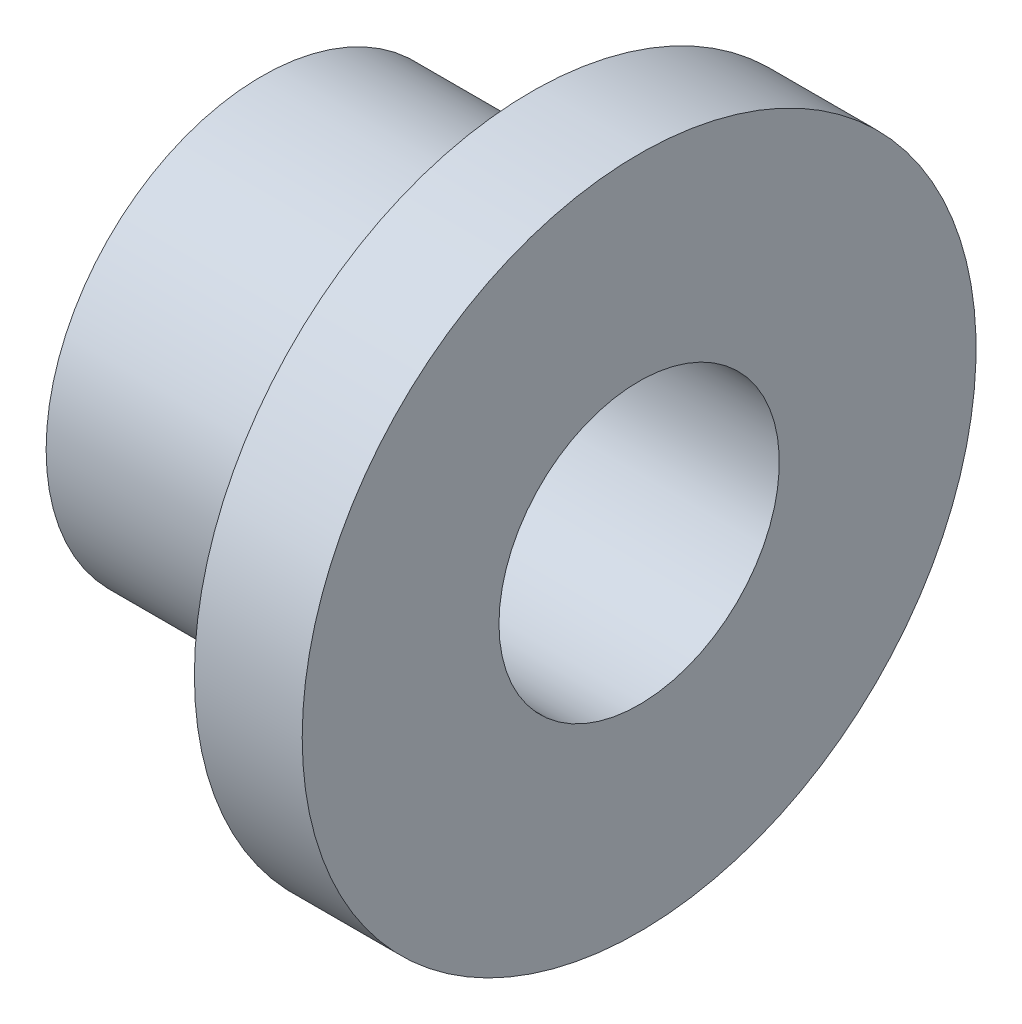
from build123d import *


with BuildPart() as part:
    # Sketch1 → Revolve1 (revolve)
    with BuildSketch(Plane.XY, mode=Mode.PRIVATE) as revolve1_sk:
        Polygon((0, -26), (0, -40), (50, -40), (50, -62.5), (70, -62.5), (70, -26), align=None)
    revolve(revolve1_sk.sketch.rotate(Axis((0, 0, 0), (1, 0, 0)), 270), axis=Axis((0, 0, 0), (1, 0, 0)))


solid = part.part
